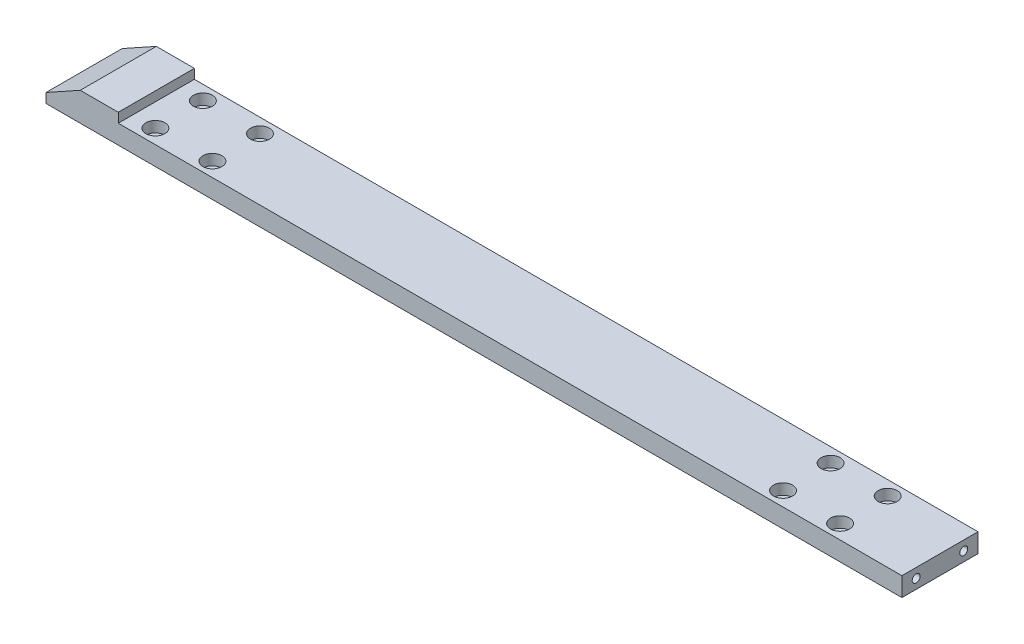
from build123d import *

# Parameters (mm, degrees)
EXTRUDE_1_DEPTH           = 20
HOLE_WIZARD_1_D           = 5.5
HOLE_WIZARD_1_DEPTH       = 14
HOLE_WIZARD_1_CBORE_D     = 10
HOLE_WIZARD_1_CBORE_DEPTH = 5.7
HOLE_WIZARD_1_TIP         = 1.652366702
HOLE_WIZARD_M5_1_D        = 4.2
HOLE_WIZARD_M5_1_DEPTH    = 14
HOLE_WIZARD_M5_1_TIP      = 1.2618073


with BuildPart() as part:
    # 草图1 → 凸台-拉伸1 (new, symmetric)
    with BuildSketch(Plane.XY):
        Polygon((0, 0), (450, 0), (450, 10), (38, 10), (38, 15), (18, 15), (0, 5), align=None)
    extrude(amount=EXTRUDE_1_DEPTH, both=True)

    # 打孔尺寸(%根据)内六角圆柱头螺钉的类型1
    with Locations(Plane(origin=(0, 10, 0), x_dir=(1, 0, 0), z_dir=(0, 1, 0))):
        with Locations((50, 12.5), (80, 12.5), (50, -12.5), (80, -12.5), (380, -12.5), (410, -12.5), (380, 12.5), (410, 12.5)):
            CounterBoreHole(HOLE_WIZARD_1_D / 2, HOLE_WIZARD_1_CBORE_D / 2, HOLE_WIZARD_1_CBORE_DEPTH, depth=HOLE_WIZARD_1_DEPTH)
            with Locations((0, 0, -(HOLE_WIZARD_1_DEPTH + HOLE_WIZARD_1_TIP / 2))):  # 118° drill point
                Cone(0, HOLE_WIZARD_1_D / 2, HOLE_WIZARD_1_TIP, mode=Mode.SUBTRACT)

    # M5 螺纹孔1
    with Locations(Plane(origin=(450, 0, 0), x_dir=(0, 0, -1), z_dir=(1, 0, 0))):
        with Locations((-12.5, 5), (12.5, 5)):
            Hole(HOLE_WIZARD_M5_1_D / 2, depth=HOLE_WIZARD_M5_1_DEPTH)
            with Locations((0, 0, -(HOLE_WIZARD_M5_1_DEPTH + HOLE_WIZARD_M5_1_TIP / 2))):  # 118° drill point
                Cone(0, HOLE_WIZARD_M5_1_D / 2, HOLE_WIZARD_M5_1_TIP, mode=Mode.SUBTRACT)


solid = part.part
